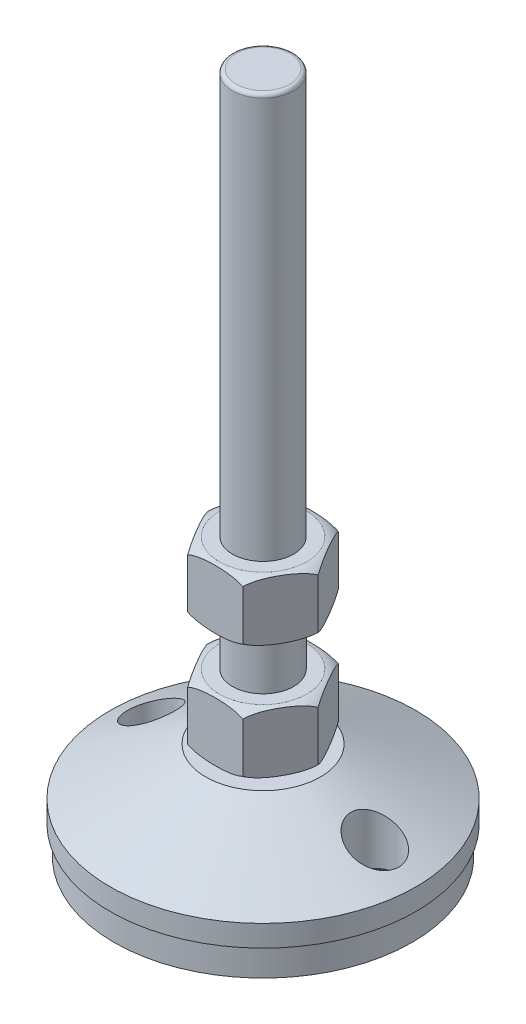
SolidWorks part; units mm, degrees
material "S45C"
ref_plane "前视基准面" through (0, 0, 0) normal (0, 0, 1) x (1, 0, 0)
ref_plane "上视基准面" through (0, 0, 0) normal (0, 1, 0) x (1, 0, 0)
ref_plane "右视基准面" through (0, 0, 0) normal (1, 0, 0) x (0, 0, -1)
sketch "草图1" plane through (0, 0, 0) normal (0, 0, 1) x (1, 0, 0)
  line L0 (0, -6.2143) -> (0, 112.5) construction
  line L1 (18.7607, 7.5) -> (13.3968, 18.8)
  line L2 (19, 0) -> (39, 0)
  line L4 (18.7607, 7.5) -> (39, 7.5)
  line L5 (39, 0) -> (39, 7.5)
  line L6 (8, 18.8) -> (8, 15.8)
  line L7 (8, 15.8) -> (11.5, 15.8)
  line L8 (11.5, 15.8) -> (19, 0)
  line L9 (8, 18.8) -> (13.3968, 18.8)
  dimension "D1" = 20
  dimension "D2" = 78
  dimension "D3" = 7.5
  dimension "D4" = 16
  dimension "D5" = 23
  dimension "D6" = 15.8
  dimension "D7" = 3
  dimension "D8" = 3
revolve "旋转1" add sketch "草图1" angle 360 about L0
hole_wizard "Ø12.0 (12) 直径孔1" positions "草图3" profile "草图4" hole size "Ø12.0" standard "GB" end condition through all
sketch "草图3" plane through (0, 7.5, 0) normal (0, 1, 0) x (1, 0, 0)
  line L0 (-49.5004, 0) -> (60.188, 0) construction
  circle A0 centre (0, 0) radius 29.25 construction
  point P0 (-29.25, 0)
  point P13 (29.25, 0)
  dimension "D1" = 58.5
sketch "草图4" plane through (-29.25, 7.5, 0) normal (1, 0, 0) x (0, 0, 1)
  line L0 (0, 0) -> (0, 7.5)
  line L1 (0, 7.5) -> (6, 7.5)
  line L2 (6, 7.5) -> (6, 0)
  line L5 (6, 0) -> (0, 0)
  line L11 (0, -6.35) -> (0, 107.95) construction
  dimension "通孔孔直径" = 12
  dimension "通孔孔深度" = 7.5
sketch "草图2" plane through (0, 0, 0) normal (0, 0, 1) x (1, 0, 0)
  line L0 (0, -3.8725) -> (0, 188.1737) construction
  line L2 (-40, 7.5) -> (-18.7607, 7.5)
  line L3 (-40, 7.5) -> (-40, 13.1)
  line L6 (-15, 25.5) -> (-40, 13.1)
  line L7 (-39, 0) -> (39, 0) construction
  line L8 (-13.3968, 18.8) -> (-18.7607, 7.5)
  line L9 (-13.3968, 18.8) -> (-8, 18.8)
  line L10 (8, 18.8) -> (-8, 18.8) construction
  line L11 (-8, 15.8) -> (-8, 18.8)
  line L12 (-8, 25.5) -> (-15, 25.5)
  line L13 (-13.3968, 18.8) -> (-18.7607, 7.5) construction
  line L14 (13.3968, 18.8) -> (-13.3968, 18.8) construction
  line L15 (-11, 8.3) -> (0, 8.3)
  line L18 (-11, 15.8) -> (-11, 8.3)
  line L19 (0, 178.5) -> (-8, 178.5)
  line L21 (-8, 15.8) -> (-11, 15.8)
  line L22 (-11.5, 15.8) -> (11.5, 15.8) construction
  line L23 (-8, 25.5) -> (-8, 178.5)
  line L24 (0, 8.3) -> (0, 178.5)
  line L25 (39, 7.5) -> (-39, 7.5) construction
  point P23 (0, 102.8056)
  dimension "D1" = 25.5
  dimension "D2" = 13.1
  dimension "D3" = 30
  dimension "D4" = 3
  dimension "D5" = 7.5
  dimension "D6" = 153
  dimension "D7" = 80
revolve "旋转2" add sketch "草图2" angle 360 about L0
cosmetic thread "装饰螺纹线1" parameters "D2"=13.835
ref_plane "基准面1" through (0, 26.5, 0) normal (0, 1, 0) x (1, 0, 0)
sketch "草图6" plane through (0, 26.5, 0) normal (0, 1, 0) x (1, 0, 0)
  line L0 (-26.6755, 0) -> (26.0956, 0) construction
  line L1 (14.4338, 0) -> (7.2169, 12.5)
  line L2 (7.2169, 12.5) -> (-7.2169, 12.5)
  line L3 (-7.2169, 12.5) -> (-14.4338, 0)
  line L4 (-14.4338, 0) -> (-7.2169, -12.5)
  line L5 (-7.2169, -12.5) -> (7.2169, -12.5)
  line L6 (7.2169, -12.5) -> (14.4338, 0)
  circle A0 centre (0, 0) radius 12.5 construction
  dimension "D1" = 25
extrude "凸台-拉伸1" add sketch "草图6" along normal blind 16
sketch "草图7" plane through (0, 0, 0) normal (0, 0, 1) x (1, 0, 0)
  line L0 (0, -6.4673) -> (0, 69.5673) construction
  line L1 (14.4338, 42.5) -> (11.4338, 42.5)
  line L2 (7.2169, 42.5) -> (14.4338, 42.5) construction
  line L3 (14.4338, 42.5) -> (14.4338, 41)
  line L4 (14.4338, 42.5) -> (14.4338, 26.5) construction
  line L5 (-14.4338, 34.5) -> (18.0107, 34.5) construction
  line L6 (-14.4338, 42.5) -> (-14.4338, 26.5) construction
  line L7 (14.4338, 26.5) -> (14.4338, 28)
  line L8 (14.4338, 26.5) -> (11.4338, 26.5)
  arc A0 (11.4338, 42.5) -> (14.4338, 41) centre (10.3574, 36.5973) cw
  arc A1 (11.4338, 26.5) -> (14.4338, 28) centre (10.3574, 32.4027) ccw
  dimension "D3" = 6
  dimension "D1" = 3
  dimension "D2" = 1.5
revolve "切除-旋转1" cut sketch "草图7" angle 360 about L0
pattern_linear "阵列(线性)1" count 2 spacing 30 along (0, 1, 0) of "凸台-拉伸1", "切除-旋转1"
hole_wizard "Ø12.5 (12.5) 直径孔1" positions "草图8" profile "草图9" hole size "Ø12.5" standard "GB" end condition through all
sketch "草图8" plane through (0, 7.5, 0) normal (0, -1, 0) x (-1, 0, 0)
  point P0 (-29.25, 0)
  point P3 (29.25, 0)
sketch "草图9" plane through (29.25, 7.5, 0) normal (1, 0, 0) x (0, 0, -1)
  line L0 (0, 0) -> (0, 171)
  line L1 (0, 171) -> (6.25, 171)
  line L2 (6.25, 171) -> (6.25, 0)
  line L5 (6.25, 0) -> (0, 0)
  line L11 (0, -6.35) -> (0, 107.95) construction
  dimension "通孔孔直径" = 12.5
  dimension "通孔孔深度" = 171
fillet "圆角1" radius 1 1 edges at (0, 178.5, -8)
